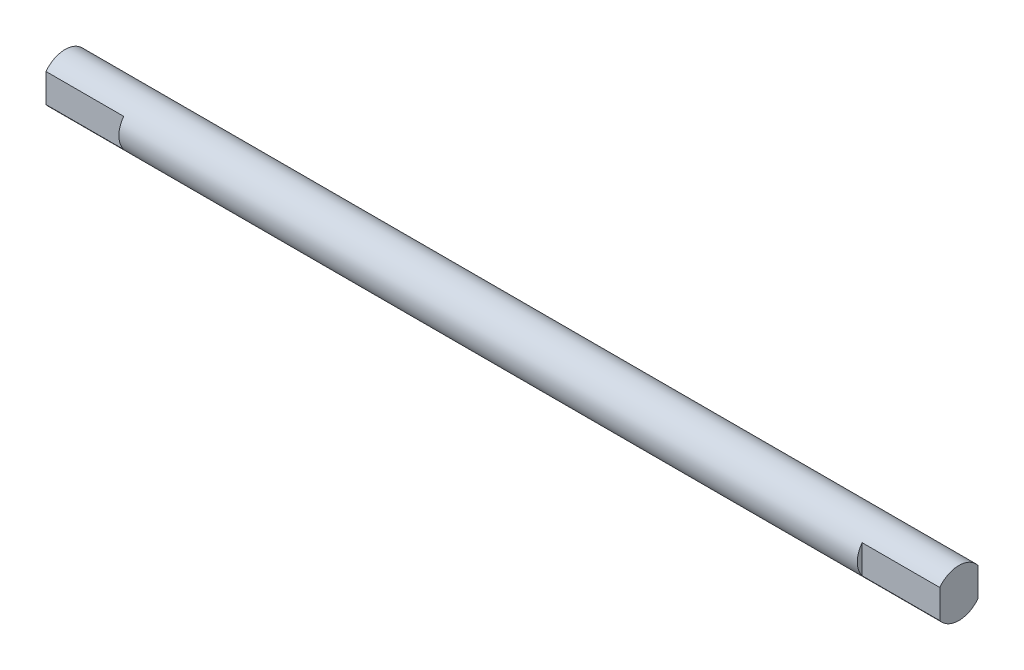
from build123d import *

# Parameters (mm, degrees)
SKETCH1_R           = 10
BOSS_EXTRUDE1_DEPTH = 374
CUT_EXTRUDE1_START  = -8
SKETCH_2_2_W        = 44.374102045
SKETCH_2_2_H        = 48.77153558
SKETCH_2_2_W_2      = 193.002207495
SKETCH_2_2_H_2      = 56.618631092
CUT_EXTRUDE1_DEPTH  = 20
CUT_EXTRUDE2_START  = 8
SKETCH_2_2_2_W      = 44.374102045
SKETCH_2_2_2_H      = 48.77153558
SKETCH_2_2_2_W_2    = 193.002207495
SKETCH_2_2_2_H_2    = 56.618631092
CUT_EXTRUDE2_DEPTH  = 20


with BuildPart() as part:
    # Sketch1 → Boss-Extrude1 (new body)
    with BuildSketch(Plane(origin=(0, 0, 0), x_dir=(0, 0, -1), z_dir=(1, 0, 0))):
        Circle(SKETCH1_R)
    extrude(amount=BOSS_EXTRUDE1_DEPTH)

    # Sketch 2_2 → Cut-Extrude1 (cut)
    with BuildSketch(Plane.XY.offset(CUT_EXTRUDE1_START)):
        with Locations((10.312948977, 5.596733591)):
            Rectangle(SKETCH_2_2_W, SKETCH_2_2_H)
        with Locations((438.001103747, 0.32564759)):
            Rectangle(SKETCH_2_2_W_2, SKETCH_2_2_H_2)
    extrude(amount=-CUT_EXTRUDE1_DEPTH, mode=Mode.SUBTRACT)

    # Sketch 2_2 2 → Cut-Extrude2 (cut)
    with BuildSketch(Plane.XY.offset(CUT_EXTRUDE2_START)):
        with Locations((10.312948977, 5.596733591)):
            Rectangle(SKETCH_2_2_2_W, SKETCH_2_2_2_H)
        with Locations((438.001103747, 0.32564759)):
            Rectangle(SKETCH_2_2_2_W_2, SKETCH_2_2_2_H_2)
    extrude(amount=CUT_EXTRUDE2_DEPTH, mode=Mode.SUBTRACT)


solid = part.part
